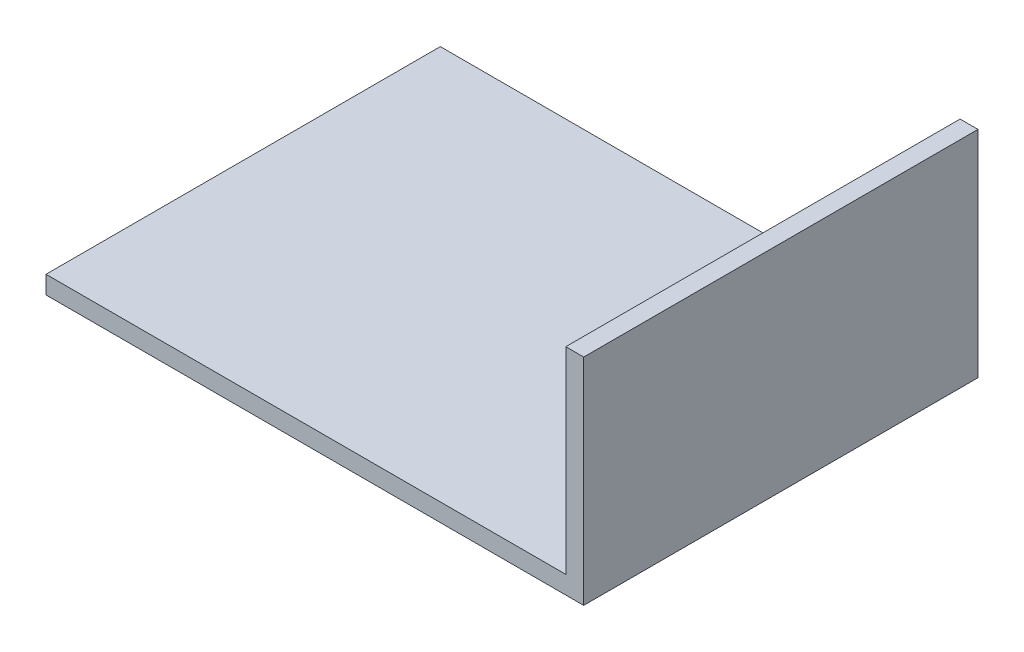
from build123d import *

# Parameters (mm, degrees)
EXTRUDE_1_DEPTH = 110


with BuildPart() as part:
    # 草图1 → 凸台-拉伸1 (new body)
    with BuildSketch(Plane.XY):
        Polygon((0, 0), (0, -60), (-150, -60), (-150, -55), (-5, -55), (-5, 0), align=None)
    extrude(amount=EXTRUDE_1_DEPTH)


solid = part.part
